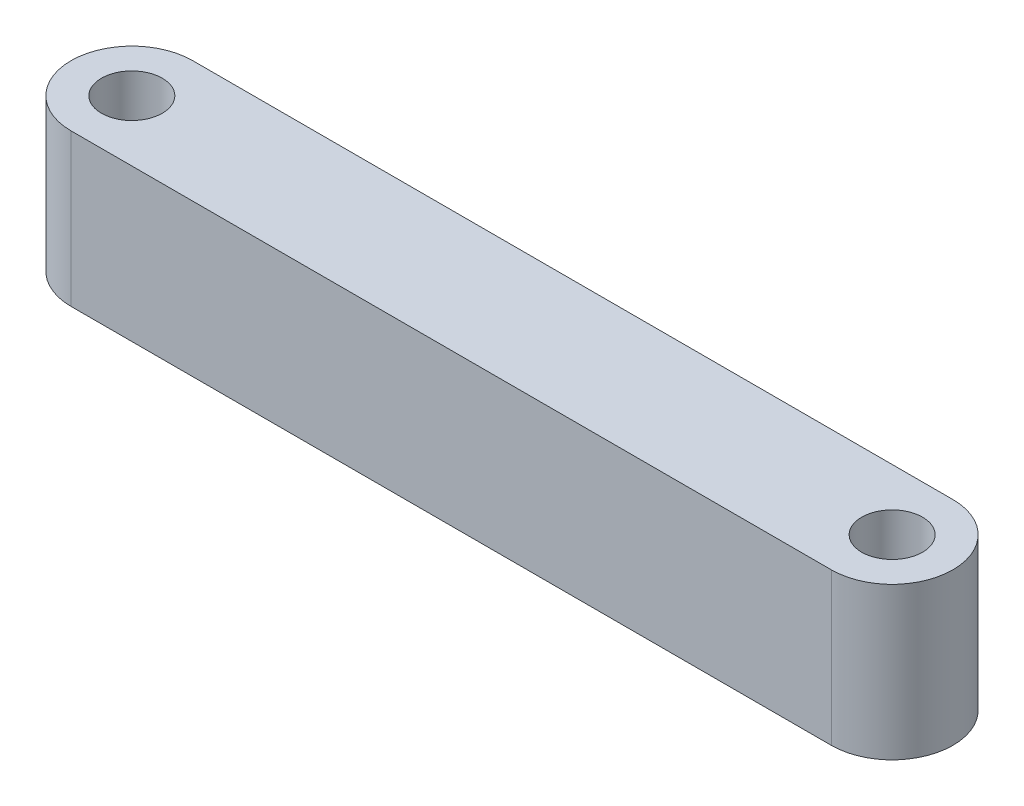
SolidWorks part; units mm, degrees
ref_plane "Front Plane" through (0, 0, 0) normal (0, 0, 1) x (1, 0, 0)
ref_plane "Top Plane" through (0, 0, 0) normal (0, 1, 0) x (1, 0, 0)
ref_plane "Right Plane" through (0, 0, 0) normal (1, 0, 0) x (0, 0, -1)
sketch "Sketch1" plane through (0, 0, 0) normal (0, 1, 0) x (1, 0, 0)
  line L0 (-25, 4) -> (25, 4)
  line L1 (25, -4) -> (-25, -4)
  line L2 (0, 39.5257) -> (0, -32.3754) construction
  line L3 (-25, 0) -> (25, 0)
  arc A0 (25, 4) -> (25, -4) centre (25, 0) cw
  arc A1 (-25, -4) -> (-25, 4) centre (-25, 0) cw
  circle A2 centre (-25, 0) radius 2
  circle A3 centre (25, 0) radius 2
  dimension "D3" = 4
  dimension "D4" = 4
  dimension "D1" = 50
  dimension "D2" = 8
extrude "Boss-Extrude1" add sketch "Sketch1" along normal blind 10
